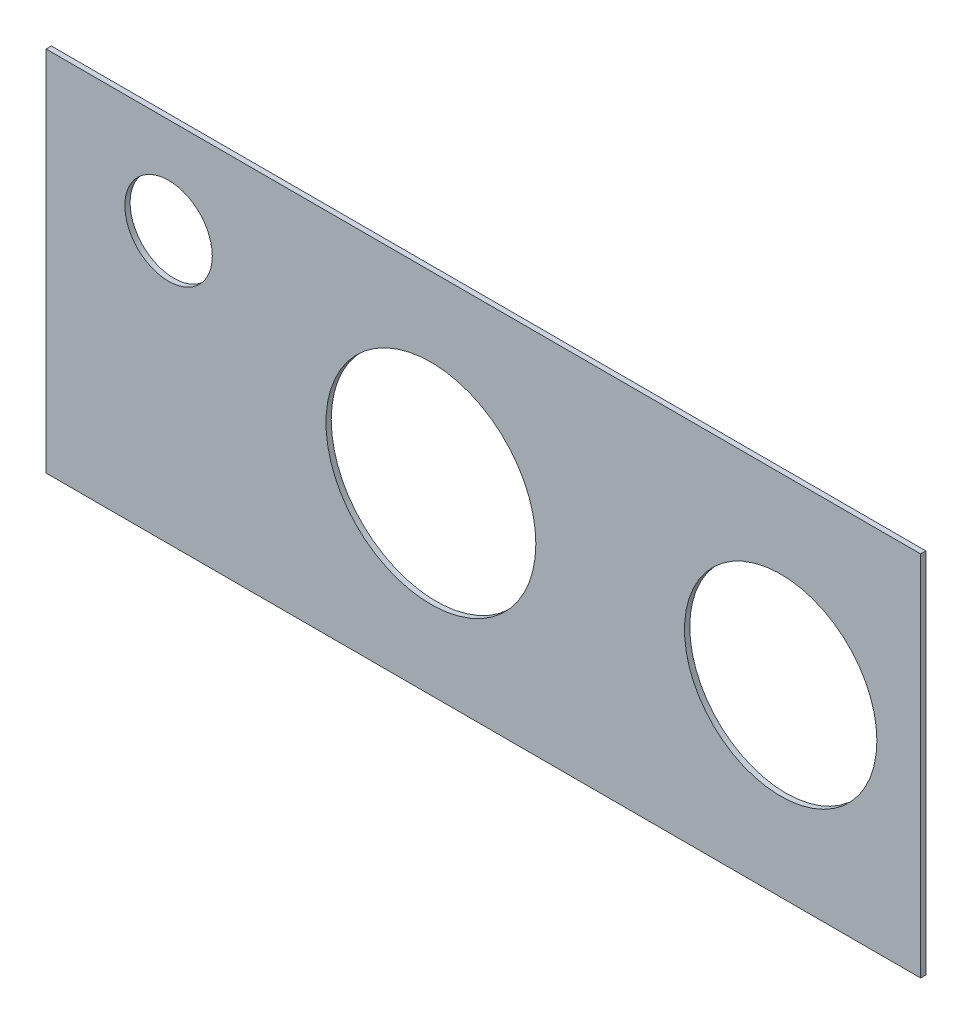
from build123d import *

# Parameters (mm, degrees)
SKETCH1_W           = 500
SKETCH1_H           = 210
BOSS_EXTRUDE1_DEPTH = 3
SKETCH2_R           = 55
SKETCH2_R_2         = 60
SKETCH2_R_3         = 25
CUT_EXTRUDE1_DEPTH  = 10


with BuildPart() as part:
    # Sketch1 → Boss-Extrude1 (new body)
    with BuildSketch(Plane.XY):
        with Locations((250, 105)):
            Rectangle(SKETCH1_W, SKETCH1_H)
    extrude(amount=BOSS_EXTRUDE1_DEPTH)

    # Sketch2 → Cut-Extrude1 (cut)
    with BuildSketch(Plane(origin=(492, 10, 3), x_dir=(1, 0, 0), z_dir=(0, 0, 1))):
        with Locations((-72, 95)):
            Circle(SKETCH2_R)
        with Locations((-272, 95)):
            Circle(SKETCH2_R_2)
        with Locations((-422, 145)):
            Circle(SKETCH2_R_3)
    extrude(amount=-CUT_EXTRUDE1_DEPTH, mode=Mode.SUBTRACT)


solid = part.part
